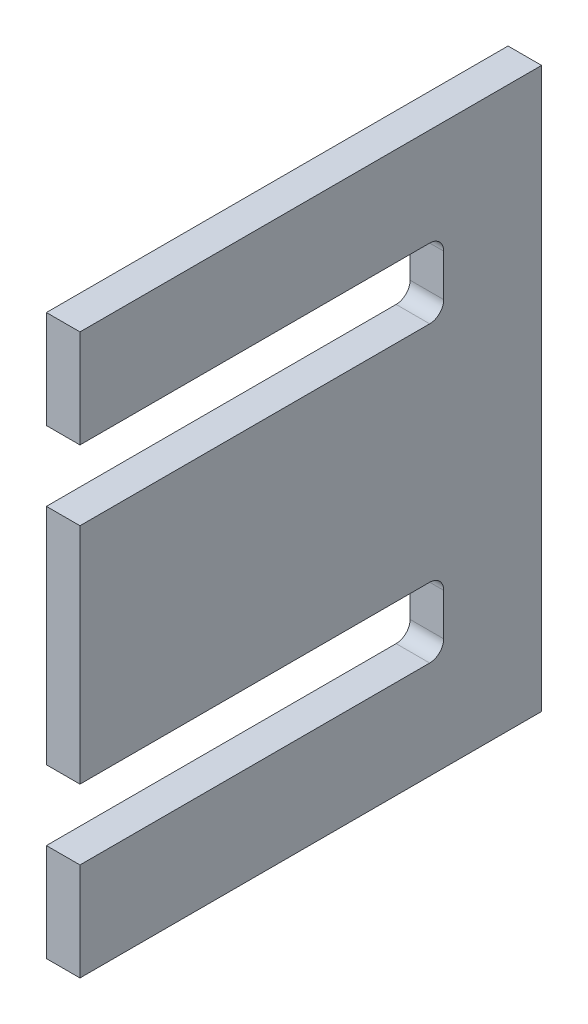
SolidWorks part; units mm, degrees
ref_plane "前视基准面" through (0, 0, 0) normal (0, 0, 1) x (1, 0, 0)
ref_plane "上视基准面" through (0, 0, 0) normal (0, 1, 0) x (1, 0, 0)
ref_plane "右视基准面" through (0, 0, 0) normal (1, 0, 0) x (0, 0, -1)
sketch "草图2" plane through (-140.7703, 0, 0) normal (-1, 0, 0) x (0, 0, 1)
  line L12 (-63, -168) -> (-63, -153)
  line L13 (-58, -148) -> (67, -148)
  line L14 (67, -148) -> (67, -68)
  line L15 (67, -68) -> (-58, -68)
  line L16 (-63, -63) -> (-63, -48)
  line L17 (-58, -43) -> (67, -43)
  line L18 (67, -43) -> (67, -8)
  line L19 (67, -8) -> (-98, -8)
  line L20 (-98, -8) -> (-98, -208)
  line L21 (-98, -208) -> (67, -208)
  line L22 (67, -208) -> (67, -173)
  line L23 (67, -173) -> (-58, -173)
  line L24 (-63, -168) -> (-63, -153)
  line L25 (-58, -148) -> (67, -148)
  line L26 (67, -148) -> (67, -68)
  line L27 (67, -68) -> (-58, -68)
  line L28 (-63, -63) -> (-63, -48)
  line L29 (-58, -43) -> (67, -43)
  line L30 (67, -43) -> (67, -8)
  line L31 (67, -8) -> (-98, -8)
  line L32 (-98, -8) -> (-98, -208)
  line L33 (-98, -208) -> (67, -208)
  line L34 (67, -208) -> (67, -173)
  line L35 (67, -173) -> (-58, -173)
  arc A4 (-58, -148) -> (-63, -153) centre (-58, -153) ccw
  arc A5 (-63, -63) -> (-58, -68) centre (-58, -63) ccw
  arc A6 (-58, -43) -> (-63, -48) centre (-58, -48) ccw
  arc A7 (-63, -168) -> (-58, -173) centre (-58, -168) ccw
  arc A8 (-58, -148) -> (-63, -153) centre (-58, -153) ccw
  arc A9 (-63, -63) -> (-58, -68) centre (-58, -63) ccw
  arc A10 (-58, -43) -> (-63, -48) centre (-58, -48) ccw
  arc A11 (-63, -168) -> (-58, -173) centre (-58, -168) ccw
  dimension "D1" = 0
extrude "凸台-拉伸1" add sketch "草图2" along normal blind 12
